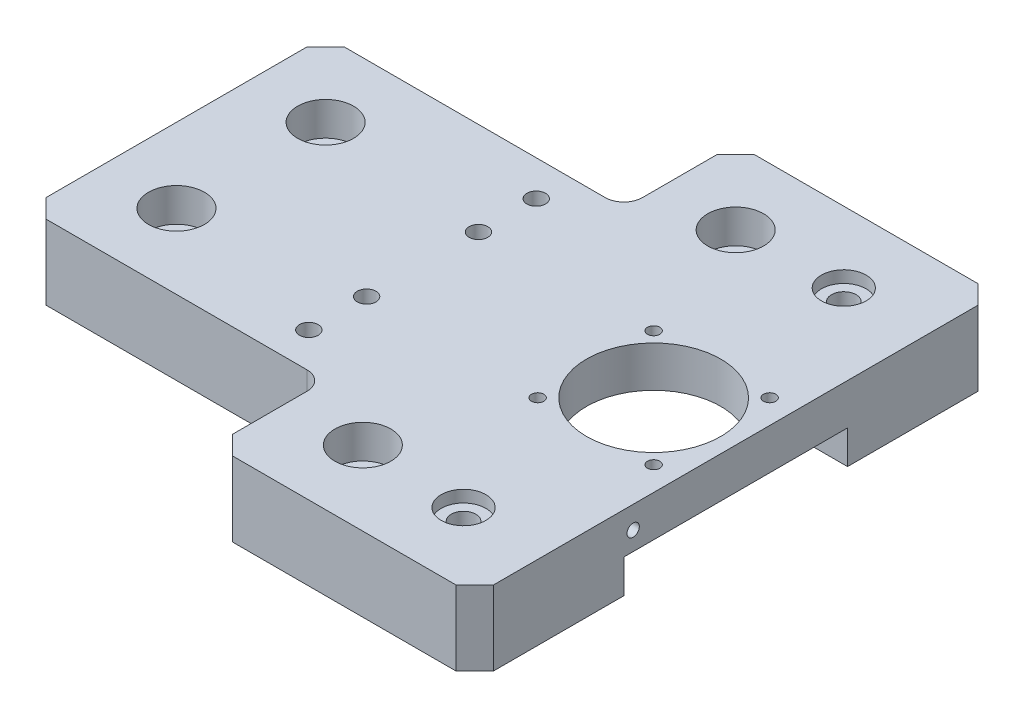
from build123d import *

# Parameters (mm, degrees)
SKETCH1_W                                            = 150
SKETCH1_H                                            = 140
BOSS_EXTRUDE1_DEPTH                                  = 20
CHAMFER1_SIZE                                        = 5
SKETCH4_R                                            = 6
CUT_EXTRUDE1_DEPTH                                   = 3.2
SKETCH7_R                                            = 18
CUT_EXTRUDE2_DEPTH                                   = 105.522724802
M4_TAPPED_HOLE1_D                                    = 3.3
SKETCH14_W                                           = 60
SKETCH14_H                                           = 9
CUT_EXTRUDE5_DEPTH                                   = 50
M4_TAPPED_HOLE3_D                                    = 3.3
M4_TAPPED_HOLE3_DEPTH                                = 11.5
M4_TAPPED_HOLE3_TIP                                  = 0.991420021
FILLET1_R                                            = 5
HOLE_SIZE_PER_SOCKET_HEAD_CAP_SCREW_TYPE_D           = 6.6
HOLE_SIZE_PER_SOCKET_HEAD_CAP_SCREW_TYPE_CBORE_D     = 11
HOLE_SIZE_PER_SOCKET_HEAD_CAP_SCREW_TYPE_CBORE_DEPTH = 6.8
SKETCH23_W                                           = 121.756161874
SKETCH23_H                                           = 40
SKETCH23_H_2                                         = 40.700827196
CUT_EXTRUDE6_DEPTH                                   = 105.522724802
FILLET2_R                                            = 5
CHAMFER2_SIZE                                        = 5
HOLE_SIZE_PER_SOCKET_HEAD_CAP_SCREW_2_D              = 9
HOLE_SIZE_PER_SOCKET_HEAD_CAP_SCREW_2_CBORE_D        = 15
HOLE_SIZE_PER_SOCKET_HEAD_CAP_SCREW_2_CBORE_DEPTH    = 9
M6_TAPPED_HOLE1_D                                    = 5
M6_TAPPED_HOLE1_DEPTH                                = 17
M6_TAPPED_HOLE1_TIP                                  = 1.502151548
BLIND_DOWEL_HOLE1_SIZE_MM_D                          = 5
BLIND_DOWEL_HOLE1_SIZE_MM_DEPTH                      = 17
BLIND_DOWEL_HOLE1_SIZE_MM_TIP                        = 1.502151548
F_6_0_6_DIAMETER_HOLE1_D                             = 6
F_6_0_6_DIAMETER_HOLE1_DEPTH                         = 17
F_6_0_6_DIAMETER_HOLE1_TIP                           = 1.802581857


with BuildPart() as part:
    # Sketch1 → Boss-Extrude1 (new body)
    with BuildSketch(Plane(origin=(0, 0, 0), x_dir=(1, 0, 0), z_dir=(0, 1, 0))):
        Rectangle(SKETCH1_W, SKETCH1_H)
    extrude(amount=BOSS_EXTRUDE1_DEPTH)

    # Chamfer1
    chamfer1_edges = [part.edges().sort_by_distance(p)[0] for p in [
        (-75, 10, -70),
        (75, 10, -70),
        (75, 10, 70),
        (-75, 10, 70),
    ]]
    chamfer(chamfer1_edges, length=CHAMFER1_SIZE)

    # Sketch4 → Cut-Extrude1 (cut)
    with BuildSketch(Plane(origin=(0, 20, 0), x_dir=(1, 0, 0), z_dir=(0, 1, 0))):
        with Locations(Location((53, -51, 0), (0, 0, 270))):
            Circle(SKETCH4_R)
        with Locations(Location((53, 51, 0), (0, 0, 90))):
            Circle(SKETCH4_R)
    extrude(amount=-CUT_EXTRUDE1_DEPTH, mode=Mode.SUBTRACT)

    # Sketch7 → Cut-Extrude2 (cut, through all)
    with BuildSketch(Plane(origin=(0, 20, 0), x_dir=(1, 0, 0), z_dir=(0, 1, 0))):
        with Locations(Location((53, 0, 0), (0, 0, 270))):
            Circle(SKETCH7_R)
    extrude(amount=-CUT_EXTRUDE2_DEPTH, mode=Mode.SUBTRACT)

    # M4 Tapped Hole1 (through all)
    with Locations(Plane(origin=(0, 20, 0), x_dir=(-1, 0, 0), z_dir=(0, 1, 0))):
        with Locations((-68.5565, 15.5565), (-68.5565, -15.5565), (-37.4435, -15.5565), (-37.4435, 15.5565)):
            Hole(M4_TAPPED_HOLE1_D / 2)

    # Sketch14 → Cut-Extrude5 (cut)
    with BuildSketch(Plane(origin=(75, 0, 0), x_dir=(0, 0, -1), z_dir=(1, 0, 0))):
        with Locations((0, 4.5)):
            Rectangle(SKETCH14_W, SKETCH14_H)
    extrude(amount=-CUT_EXTRUDE5_DEPTH, mode=Mode.SUBTRACT)

    # M4 Tapped Hole3
    with Locations(Plane(origin=(75, 0, 0), x_dir=(0, 0, -1), z_dir=(1, 0, 0))):
        with Locations((-27.5, 14)):
            Hole(M4_TAPPED_HOLE3_D / 2, depth=M4_TAPPED_HOLE3_DEPTH)
            with Locations((0, 0, -(M4_TAPPED_HOLE3_DEPTH + M4_TAPPED_HOLE3_TIP / 2))):  # 118° drill point
                Cone(0, M4_TAPPED_HOLE3_D / 2, M4_TAPPED_HOLE3_TIP, mode=Mode.SUBTRACT)

    # Fillet1
    fillet1_edges = [part.edges().sort_by_distance(p)[0] for p in [
        (25, 4.5, 30),
        (25, 4.5, -30),
    ]]
    fillet(fillet1_edges, radius=FILLET1_R)

    # Hole size per socket head cap screw type (through all)
    with Locations(Plane(origin=(0, 0, 0), x_dir=(-1, 0, 0), z_dir=(0, -1, 0))):
        with Locations((-53, -51), (-53, 51)):
            CounterBoreHole(HOLE_SIZE_PER_SOCKET_HEAD_CAP_SCREW_TYPE_D / 2, HOLE_SIZE_PER_SOCKET_HEAD_CAP_SCREW_TYPE_CBORE_D / 2, HOLE_SIZE_PER_SOCKET_HEAD_CAP_SCREW_TYPE_CBORE_DEPTH)

    # Sketch23 → Cut-Extrude6 (cut, through all)
    with BuildSketch(Plane(origin=(0, 20, 0), x_dir=(1, 0, 0), z_dir=(0, 1, 0))):
        with Locations((-55.878080937, 60)):
            Rectangle(SKETCH23_W, SKETCH23_H)
        with Locations((-55.878080937, -60.350413598)):
            Rectangle(SKETCH23_W, SKETCH23_H_2)
    extrude(amount=-CUT_EXTRUDE6_DEPTH, mode=Mode.SUBTRACT)

    # Fillet2
    fillet2_edges = [part.edges().sort_by_distance(p)[0] for p in [
        (5, 10, -40),
        (5, 10, 40),
    ]]
    fillet(fillet2_edges, radius=FILLET2_R)

    # Chamfer2
    chamfer2_edges = [part.edges().sort_by_distance(p)[0] for p in [
        (5, 10, -70),
        (-75, 10, -40),
        (5, 10, 70),
        (-75, 10, 40),
    ]]
    chamfer(chamfer2_edges, length=CHAMFER2_SIZE)

    # Hole size per socket head cap screw  2 (through all)
    with Locations(Plane(origin=(0, 20, 0), x_dir=(1, 0, 0), z_dir=(0, 1, 0))):
        with Locations((25, 50), (25, -50), (-55, 20), (-55, -20)):
            CounterBoreHole(HOLE_SIZE_PER_SOCKET_HEAD_CAP_SCREW_2_D / 2, HOLE_SIZE_PER_SOCKET_HEAD_CAP_SCREW_2_CBORE_D / 2, HOLE_SIZE_PER_SOCKET_HEAD_CAP_SCREW_2_CBORE_DEPTH)

    # M6 Tapped Hole1
    with Locations(Plane(origin=(0, 20, 0), x_dir=(1, 0, 0), z_dir=(0, 1, 0))):
        with Locations((-9, 30.5), (-9, -30.5)):
            Hole(M6_TAPPED_HOLE1_D / 2, depth=M6_TAPPED_HOLE1_DEPTH)
            with Locations((0, 0, -(M6_TAPPED_HOLE1_DEPTH + M6_TAPPED_HOLE1_TIP / 2))):  # 118° drill point
                Cone(0, M6_TAPPED_HOLE1_D / 2, M6_TAPPED_HOLE1_TIP, mode=Mode.SUBTRACT)

    # Blind dowel hole1, size mm
    with Locations(Plane(origin=(0, 20, 0), x_dir=(-1, 0, 0), z_dir=(0, 1, 0))):
        with Locations((9, -15), (9, 15)):
            Hole(BLIND_DOWEL_HOLE1_SIZE_MM_D / 2, depth=BLIND_DOWEL_HOLE1_SIZE_MM_DEPTH)
            with Locations((0, 0, -(BLIND_DOWEL_HOLE1_SIZE_MM_DEPTH + BLIND_DOWEL_HOLE1_SIZE_MM_TIP / 2))):  # 118° drill point
                Cone(0, BLIND_DOWEL_HOLE1_SIZE_MM_D / 2, BLIND_DOWEL_HOLE1_SIZE_MM_TIP, mode=Mode.SUBTRACT)

    # Ø6.0 (6) Diameter Hole1
    with Locations(Plane(origin=(0, 0, 0), x_dir=(-1, 0, 0), z_dir=(0, -1, 0))):
        with Locations((55, 0), (-15, 0)):
            Hole(F_6_0_6_DIAMETER_HOLE1_D / 2, depth=F_6_0_6_DIAMETER_HOLE1_DEPTH)
            with Locations((0, 0, -(F_6_0_6_DIAMETER_HOLE1_DEPTH + F_6_0_6_DIAMETER_HOLE1_TIP / 2))):  # 118° drill point
                Cone(0, F_6_0_6_DIAMETER_HOLE1_D / 2, F_6_0_6_DIAMETER_HOLE1_TIP, mode=Mode.SUBTRACT)


solid = part.part
